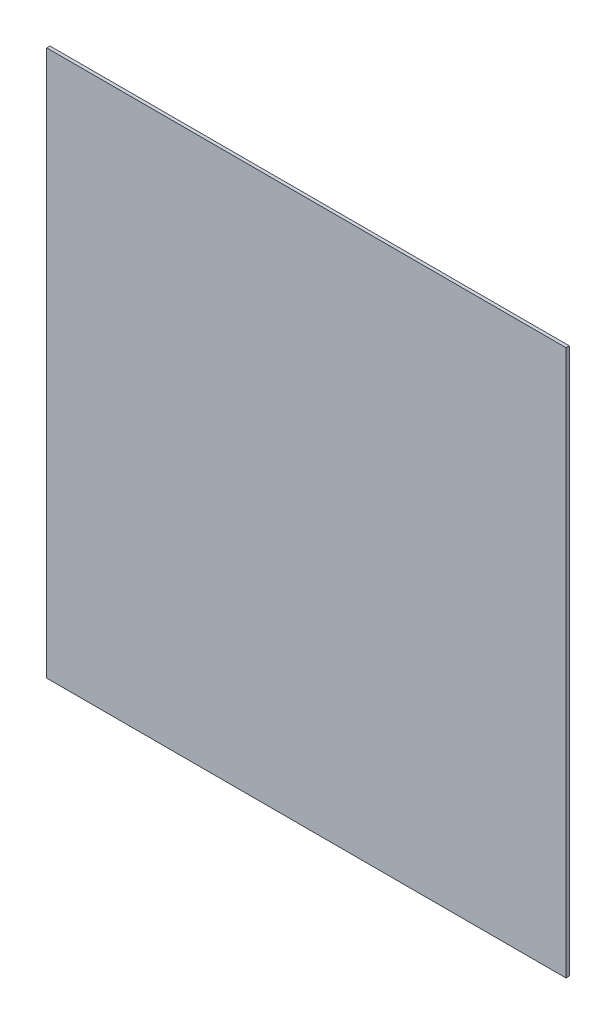
from build123d import *

# Parameters (mm, degrees)
SKETCH_1_W      = 801
SKETCH_1_H      = 842
EXTRUDE_1_DEPTH = 5


with BuildPart() as part:
    # 草图1 → 凸台-拉伸1 (new body)
    with BuildSketch(Plane.XY):
        Rectangle(SKETCH_1_W, SKETCH_1_H)
    extrude(amount=EXTRUDE_1_DEPTH)


solid = part.part
